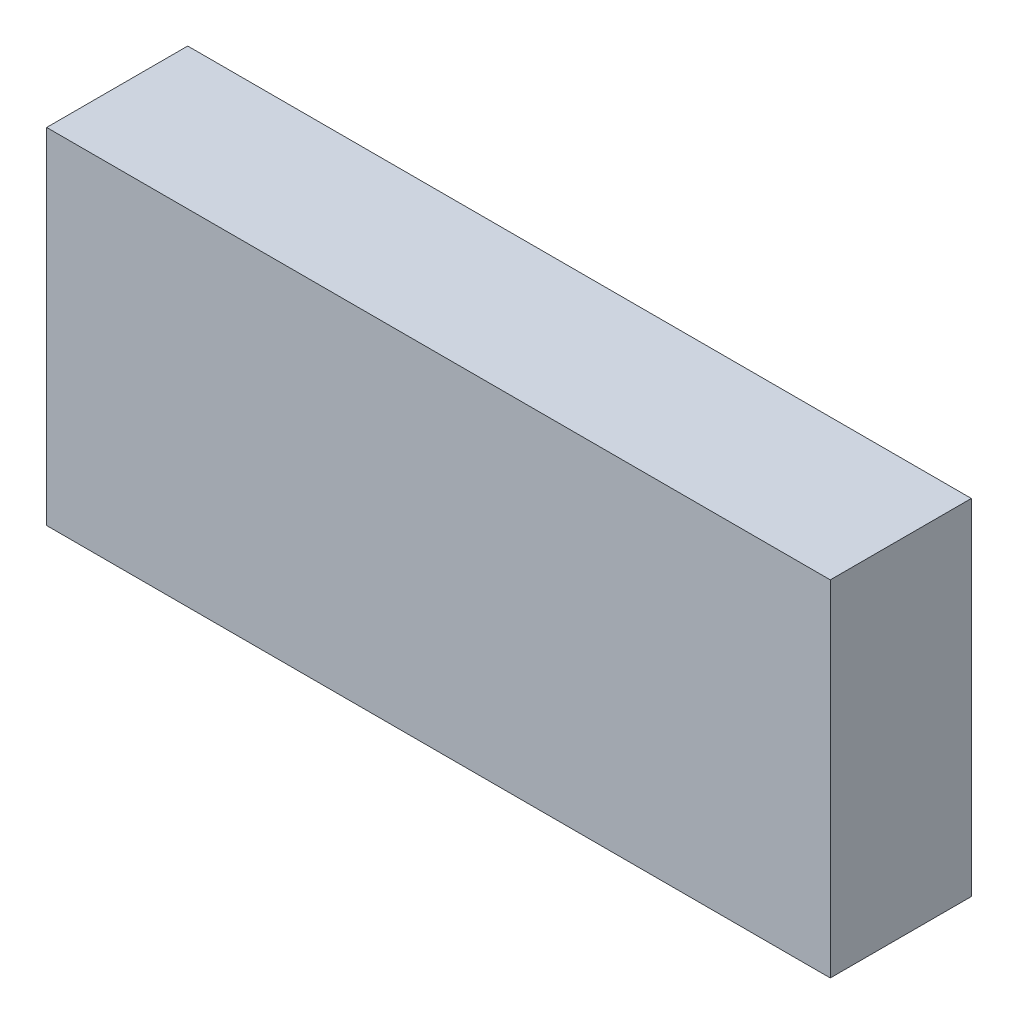
from build123d import *

# Parameters (mm, degrees)
SKETCH1_W           = 250
SKETCH1_H           = 110
BOSS_EXTRUDE1_DEPTH = 22.5


with BuildPart() as part:
    # Sketch1 → Boss-Extrude1 (new, symmetric)
    with BuildSketch(Plane.XY):
        Rectangle(SKETCH1_W, SKETCH1_H)
    extrude(amount=BOSS_EXTRUDE1_DEPTH, both=True)


solid = part.part
